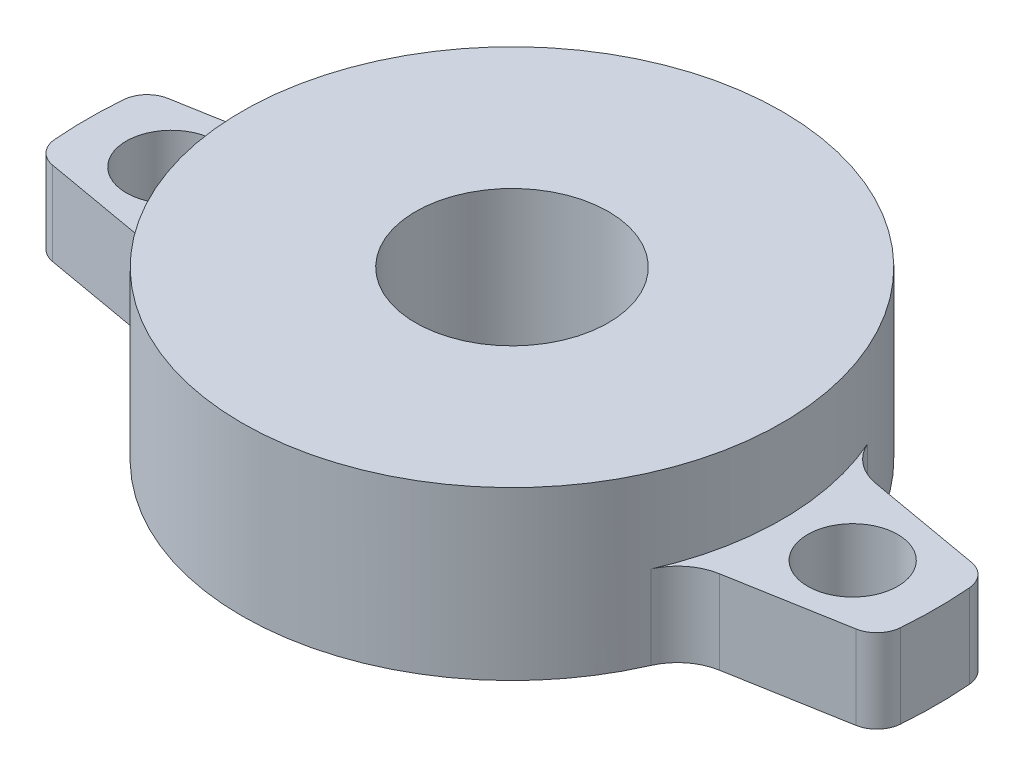
from build123d import *

# Parameters (mm, degrees)
SKETCH_1_R          = 21
SKETCH_1_R_2        = 7.5
EXTRUDE_1_DEPTH     = 13
EXTRUDE_2_DEPTH     = 6.5
FILLET_1_R          = 4
FILLET_2_R          = 2
SKETCH_3_R          = 3.5
CUT_EXTRUDE_1_DEPTH = 6.5
SKETCH_4_R          = 18
CUT_EXTRUDE_2_DEPTH = 2


with BuildPart() as part:
    # 草图1 → 凸台-拉伸1 (new body)
    with BuildSketch(Plane(origin=(0, 0, 0), x_dir=(1, 0, 0), z_dir=(0, 1, 0))):
        with Locations(Location((0, 0, 0), (0, 0, 90))):
            Circle(SKETCH_1_R)
        with Locations(Location((0, 0, 0), (0, 0, 90))):
            Circle(SKETCH_1_R_2, mode=Mode.SUBTRACT)
    extrude(amount=EXTRUDE_1_DEPTH)

    # 草图2 → 凸台-拉伸2 (add)
    with BuildSketch(Plane.XZ):
        with BuildLine():
            Line((32.727876998, 4.229192264), (19.975971523, 6.477697255))
            ThreePointArc((19.975971523, 6.477697255), (21, 0), (19.975971523, -6.477697255))
            Line((19.975971523, -6.477697255), (32.727876998, -4.229192264))
            ThreePointArc((32.727876998, -4.229192264), (33, 0), (32.727876998, 4.229192264))
        make_face()
        with BuildLine():
            Line((-32.727876998, -4.229192264), (-19.975971523, -6.477697255))
            ThreePointArc((-19.975971523, -6.477697255), (-21, 0), (-19.975971523, 6.477697255))
            Line((-19.975971523, 6.477697255), (-32.727876998, 4.229192264))
            ThreePointArc((-32.727876998, 4.229192264), (-33, 0), (-32.727876998, -4.229192264))
        make_face()
    extrude(amount=-EXTRUDE_2_DEPTH)

    # 圆角1
    fillet_1_edges = [part.edges().sort_by_distance(p)[0] for p in [
        (19.975971523, 3.25, -6.477697255),
        (19.975971523, 3.25, 6.477697255),
        (-19.975971523, 3.25, 6.477697255),
        (-19.975971523, 3.25, -6.477697255),
    ]]
    fillet(fillet_1_edges, radius=FILLET_1_R)

    # 圆角2
    fillet_2_edges = [part.edges().sort_by_distance(p)[0] for p in [
        (32.727876998, 3.25, 4.229192264),
        (32.727876998, 3.25, -4.229192264),
        (-32.727876998, 3.25, -4.229192264),
        (-32.727876998, 3.25, 4.229192264),
    ]]
    fillet(fillet_2_edges, radius=FILLET_2_R)

    # 草图3 → 切除-拉伸1 (cut)
    with BuildSketch(Plane(origin=(0, 6.5, 0), x_dir=(1, 0, 0), z_dir=(0, 1, 0))):
        with Locations(Location((-26.5, 0, 0), (0, 0, 270))):
            Circle(SKETCH_3_R)
        with Locations(Location((26.5, 0, 0), (0, 0, 270))):
            Circle(SKETCH_3_R)
    extrude(amount=-CUT_EXTRUDE_1_DEPTH, mode=Mode.SUBTRACT)

    # 草图4 → 切除-拉伸2 (cut)
    with BuildSketch(Plane.XZ):
        with Locations(Location((0, 0, 0), (0, 0, 270))):
            Circle(SKETCH_4_R)
    extrude(amount=-CUT_EXTRUDE_2_DEPTH, mode=Mode.SUBTRACT)


solid = part.part
